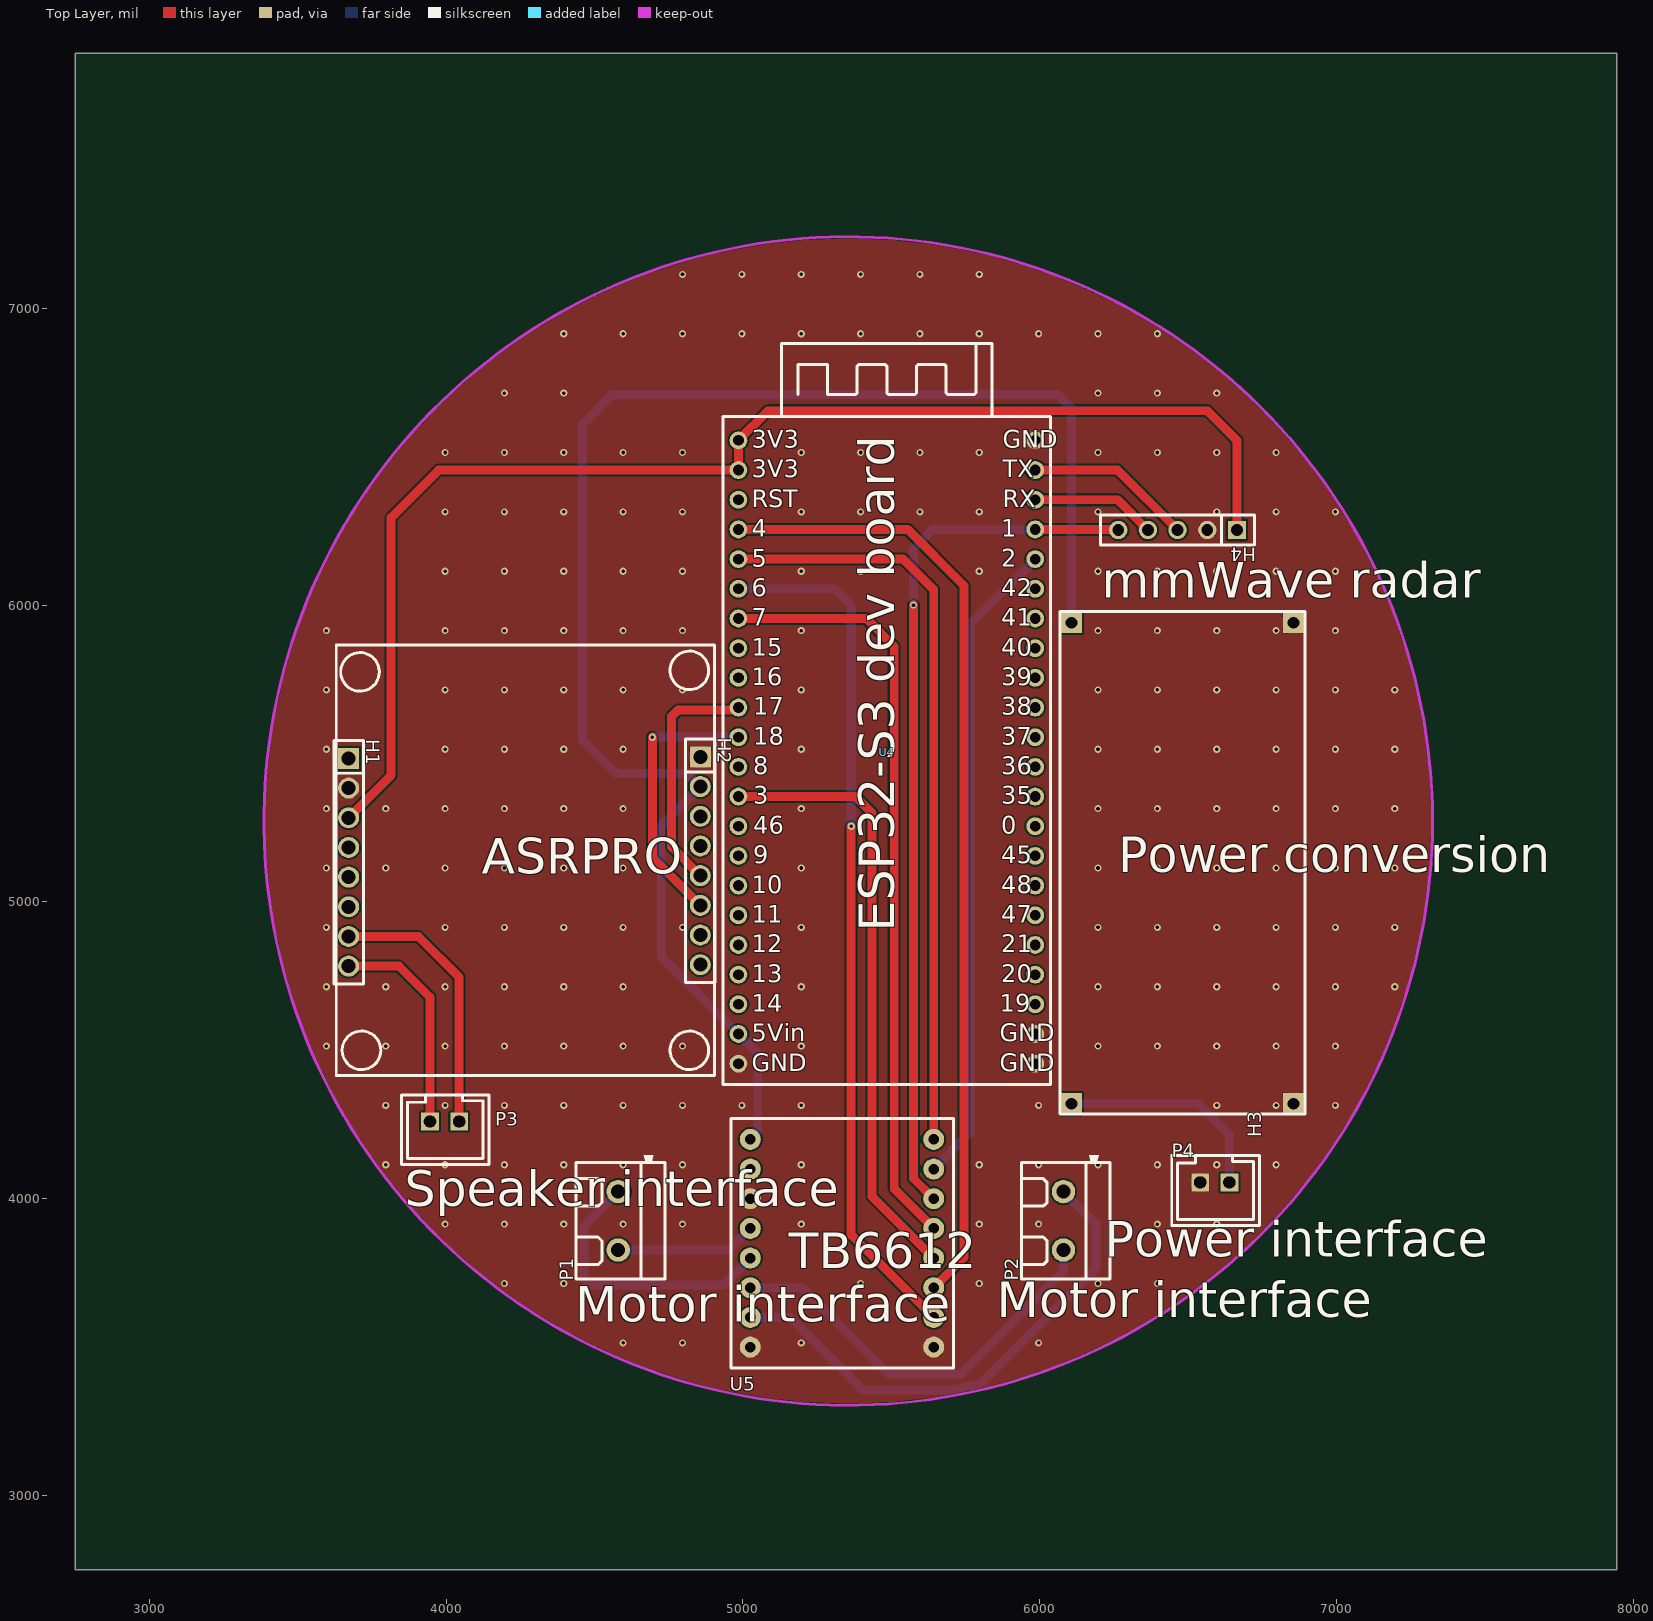
[diagram p0: Top Layer view]
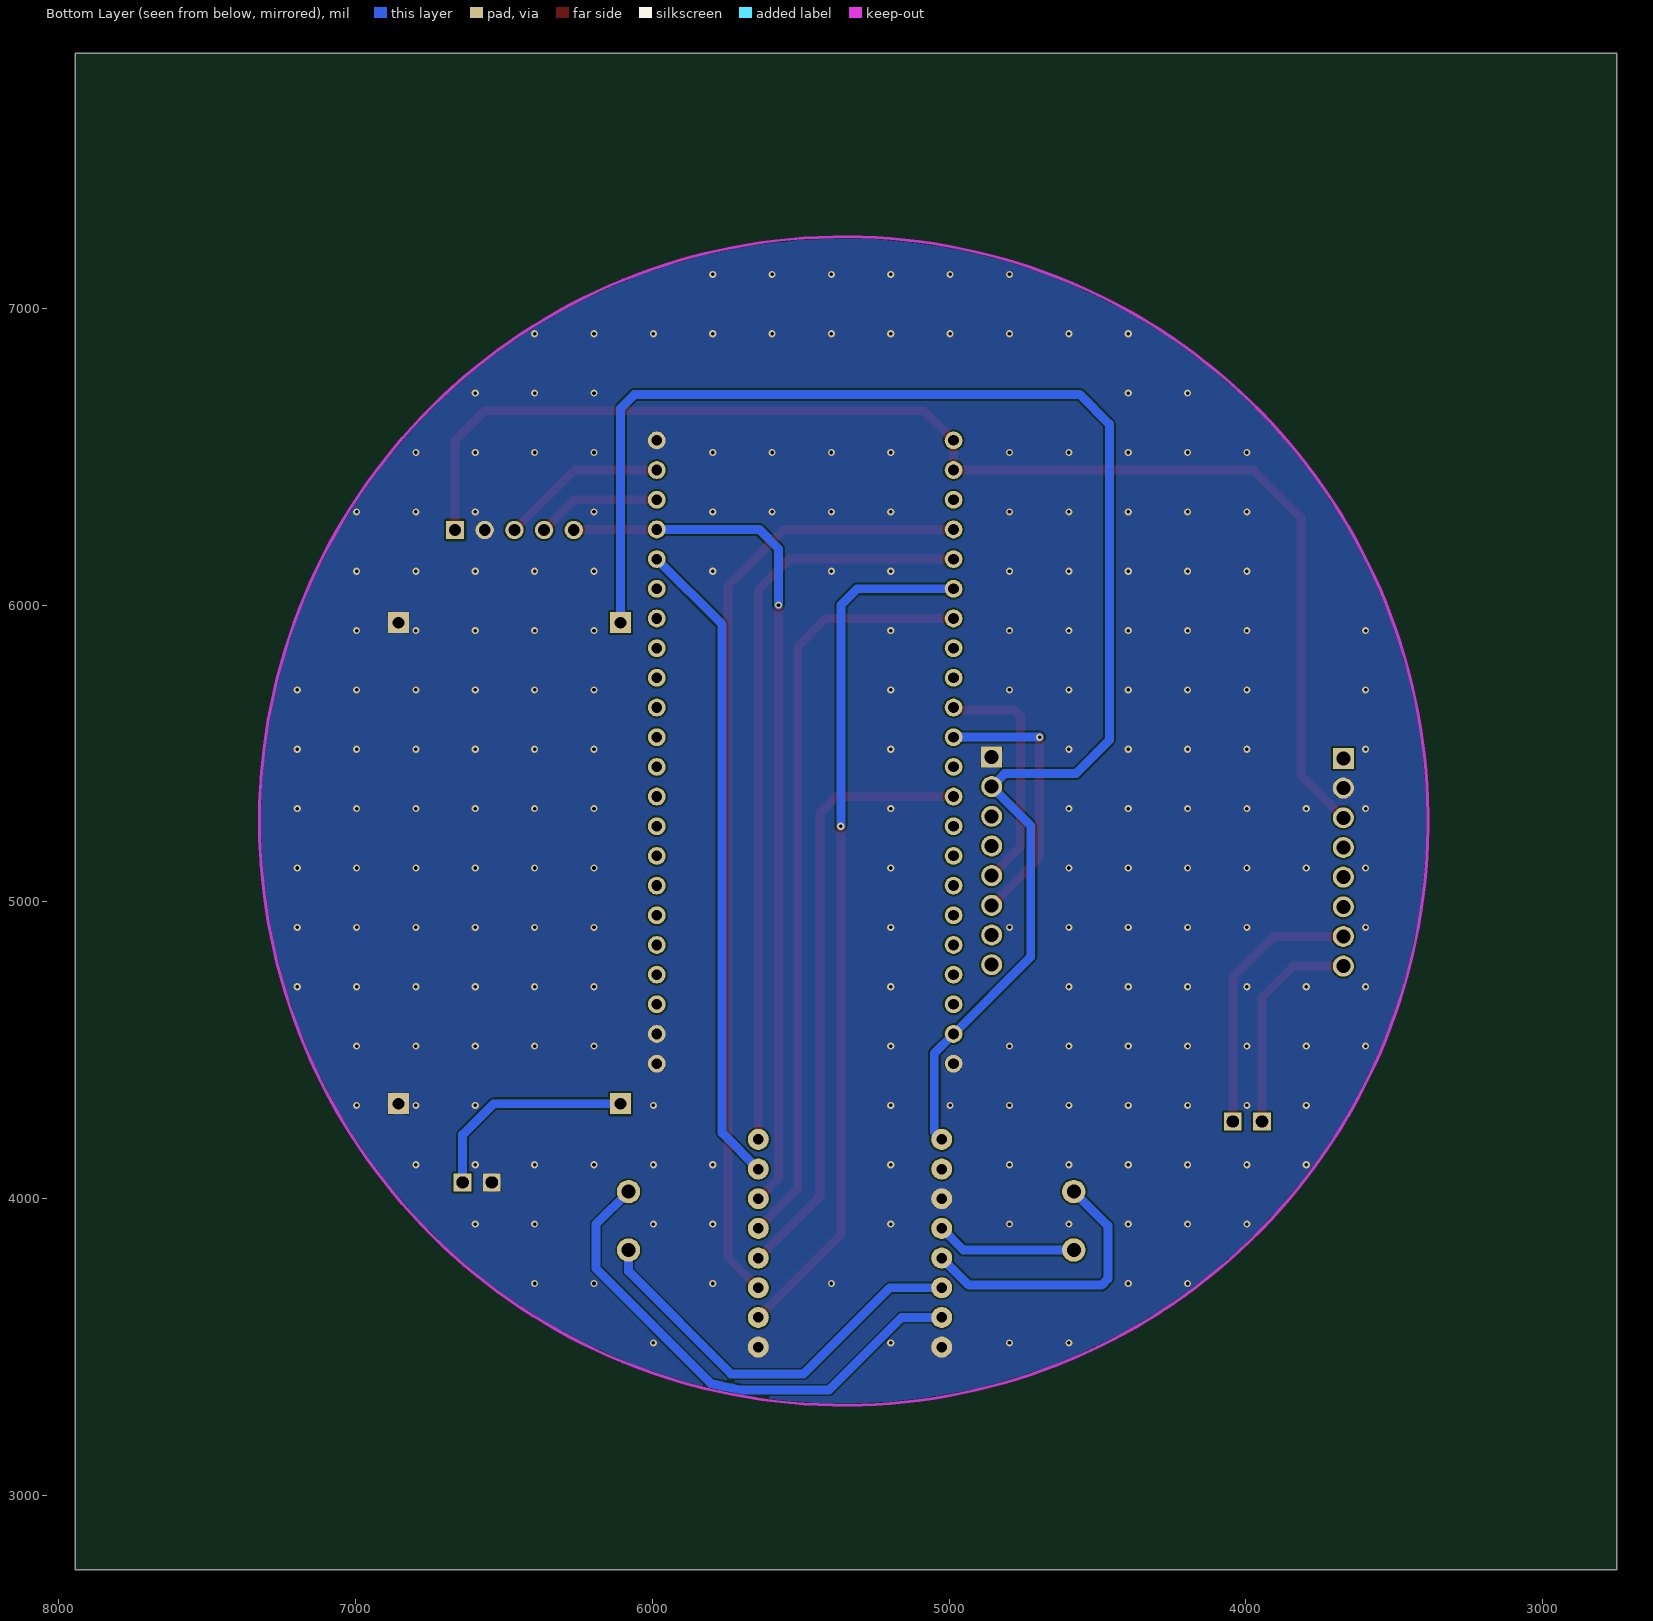
[diagram p1: Bottom Layer view, seen from below]
# Altium PCB MISC89096.pcbdoc
Units mil, origin at the board's own origin, x right, y up, seen from the top; angles counter-clockwise.
Board outline 5195 x 5110 mil, 2 copper layers (Top Layer, Bottom Layer), stack 62.206 mil thick; 10 components, 47 nets, 93 pads, 211 vias.

## Layer stack, top to bottom
Top Solder Mask Layer: solder mask 0.394, Dk 3.3
Top Layer: signal copper 1.379
Dielectric1: surface 59.449, FR4, Dk 4.5
Bottom Layer: signal copper 1.378
Bottom Solder Mask Layer: solder mask 0.394, Dk 3.3

## Board outline
7945,2750 2750,2750 2750,7860 7945,7860

## Design rules (kind name [scope] priority, off if disabled: settings)
BoardOutlineClearance Plane_Default_1 [All] p2 off: genericclearance=6 ignorepadtopadclearanceinfootprint=FALSE except(0: Arc-SplitContinuation Track-SplitContinuation SMDPad-SplitContinuation THPad-SplitContinuation Via-SplitContinuation Fill-SplitContinuation Region-SplitContinuation Poly-SplitContinuation Text-SplitContinuation Hole-SplitContinuation; 6: Arc-OutlineEdge Track-OutlineEdge SMDPad-OutlineEdge THPad-OutlineEdge Via-OutlineEdge Fill-OutlineEdge Region-OutlineEdge Poly-OutlineEdge Text-OutlineEdge Hole-OutlineEdge Arc-CutoutEdge Track-CutoutEdge SMDPad-CutoutEdge THPad-CutoutEdge Via-CutoutEdge Fill-CutoutEdge Region-CutoutEdge Poly-CutoutEdge Text-CutoutEdge Hole-CutoutEdge)
BoardOutlineClearance Copper_Default_1 [All] p4 off: genericclearance=6 ignorepadtopadclearanceinfootprint=FALSE except(0: Arc-SplitContinuation Track-SplitContinuation SMDPad-SplitContinuation THPad-SplitContinuation Via-SplitContinuation Fill-SplitContinuation Region-SplitContinuation Poly-SplitContinuation Text-SplitContinuation Hole-SplitContinuation; 6: Arc-OutlineEdge Track-OutlineEdge SMDPad-OutlineEdge THPad-OutlineEdge Via-OutlineEdge Fill-OutlineEdge Region-OutlineEdge Poly-OutlineEdge Text-OutlineEdge Hole-OutlineEdge Arc-CutoutEdge Track-CutoutEdge SMDPad-CutoutEdge THPad-CutoutEdge Via-CutoutEdge Fill-CutoutEdge Region-CutoutEdge Poly-CutoutEdge Text-CutoutEdge Hole-CutoutEdge)
BoardOutlineClearance Copper_gge24019_1 [All] p6 off: genericclearance=6 ignorepadtopadclearanceinfootprint=FALSE except(0: Arc-SplitContinuation Track-SplitContinuation SMDPad-SplitContinuation THPad-SplitContinuation Via-SplitContinuation Fill-SplitContinuation Region-SplitContinuation Poly-SplitContinuation Text-SplitContinuation Hole-SplitContinuation; 6: Arc-OutlineEdge Track-OutlineEdge SMDPad-OutlineEdge THPad-OutlineEdge Via-OutlineEdge Fill-OutlineEdge Region-OutlineEdge Text-OutlineEdge Hole-OutlineEdge Arc-CutoutEdge Track-CutoutEdge SMDPad-CutoutEdge THPad-CutoutEdge Via-CutoutEdge Fill-CutoutEdge Region-CutoutEdge Text-CutoutEdge Hole-CutoutEdge; 10: Poly-OutlineEdge Poly-CutoutEdge)
BoardOutlineClearance Default_1 [All] p8: genericclearance=6 ignorepadtopadclearanceinfootprint=FALSE except(0: Arc-SplitContinuation Track-SplitContinuation SMDPad-SplitContinuation THPad-SplitContinuation Via-SplitContinuation Fill-SplitContinuation Region-SplitContinuation Poly-SplitContinuation Text-SplitContinuation Hole-SplitContinuation; 6: Arc-OutlineEdge Track-OutlineEdge SMDPad-OutlineEdge THPad-OutlineEdge Via-OutlineEdge Fill-OutlineEdge Region-OutlineEdge Poly-OutlineEdge Text-OutlineEdge Hole-OutlineEdge Arc-CutoutEdge Track-CutoutEdge SMDPad-CutoutEdge THPad-CutoutEdge Via-CutoutEdge Fill-CutoutEdge Region-CutoutEdge Poly-CutoutEdge Text-CutoutEdge Hole-CutoutEdge)
Clearance Plane_Default [All] p1 off: gap=6 ignorepadtopadclearanceinfootprint=FALSE
Clearance Copper_Default [All] p3 off: gap=6 ignorepadtopadclearanceinfootprint=FALSE
Clearance Copper_gge24019 [All] p5 off: gap=6 ignorepadtopadclearanceinfootprint=FALSE except(10: Poly-Track Poly-SMDPad Poly-THPad Poly-Via Poly-Fill Poly-Region Poly-Poly Poly-Arc Poly-Text Poly-Hole)
Clearance Default [All] p7: gap=6 ignorepadtopadclearanceinfootprint=FALSE
DiffPairsRouting differentialPair [All] p1: maxlimit=6 minlimit=6 mostfreqgap=6 toplayer_minwidth=5 toplayer_prefwidth=10 toplayer_maxwidth=100 toplayer_mingap=6 toplayer_prefgap=6 toplayer_maxgap=6 bottomlayer_minwidth=5 bottomlayer_prefwidth=10 bottomlayer_maxwidth=100 bottomlayer_mingap=6 bottomlayer_prefgap=6 bottomlayer_maxgap=6 maxuncoupledlength=10
HoleToHoleClearance otherClearance [All] p1: gap=11.8 allowstackedmicrovias=TRUE
Length netLength [All] p1: minlimit=0 maxlimit=0
MatchedLengths netLengthTolerance [All] p1: tolerance=1000
PasteMaskExpansion Common [All] p1: expansion=0
PlaneConnect Default_4 [All] p1: planeconnectstyle=Relief reliefexpansion=20 reliefentries=4 reliefconductorwidth=0 reliefairgap=10
PolygonConnect gge24019 [All] p1 off: connectstyle=Relief reliefconductorwidth=0 reliefentries=4 polygonreliefangle="90 Angle" airgapwidth=1 smdpad.connectstyle=Relief smdpad.reliefconductorwidth=0 smdpad.reliefentries=4 smdpad.polygonreliefangle="90 Angle" smdpad.airgapwidth=10 via.connectstyle=Relief via.reliefconductorwidth=10 via.reliefentries=4 via.polygonreliefangle="90 Angle" via.airgapwidth=10
PolygonConnect Default_5 [All] p2: connectstyle=Relief reliefconductorwidth=0 reliefentries=4 polygonreliefangle="90 Angle" airgapwidth=1 smdpad.connectstyle=Relief smdpad.reliefconductorwidth=0 smdpad.reliefentries=4 smdpad.polygonreliefangle="90 Angle" smdpad.airgapwidth=10 via.connectstyle=Relief via.reliefconductorwidth=10 via.reliefentries=4 via.polygonreliefangle="90 Angle" via.airgapwidth=10
RoutingVias Default_3 [All] p1: holewidth=12 width=24 viastyle="Through Hole" minholewidth=12 minwidth=24 maxholewidth=2362 maxwidth=3938
SolderMaskExpansion Common_1 [IsVia] p1: expansion=-1000 istentingtop=TRUE
SolderMaskExpansion Common_1 [All] p2: expansion=2 istentingtop=FALSE
Width Default_2 [All] p1: maxlimit=10 minlimit=10 preferedwidth=10 toplayer_minwidth=10 toplayer_maxwidth=1000 toplayer_prefwidth=10 bottomlayer_minwidth=10 bottomlayer_maxwidth=1000 bottomlayer_prefwidth=10

## Components (designator, comment, footprint, x,y, rotation, side; value= is the part's Value field where it differs from the comment)
H1 "" HDR-TH_8P-P2.54-V-F-1 3671.85,5133.49 r270 top
H2 "" HDR-TH_8P-P2.54-V-F-1 4856.65,5138.49 r270 top
H3 "" HDR-TH_4P-P2.54-V-F-R2-C2-S2.54 6855,4320 r90 top
H4 "" HDR-TH_5P-P2.54-V-F 6464.74,6253.05 r180 top
P1 "KF301-2P terminal block" CONN-TH_XY301V-A-5.0-2P 4580,3925.64 r90 top
P2 "KF301-2P terminal block" CONN-TH_XY301V-A-5.0-2P 6080.18,3925.64 r90 top
P3 "XH2.54 straight socket-2P" CONN-TH_XH2.54-2P 3995,4260 r180 top
P4 "XH2.54 straight socket-2P" CONN-TH_XH2.54-2P 6590,4055 r180 top
U4 "NO" ESP32S3 5485,5510 r0 top
U5 "" tb6612 5025,4200 r0 top

## Footprints (in the part's own frame and the unit in brackets; to place one, negate y for a bottom-side part, rotate by r counter-clockwise, add the part's x,y. Pads: shape width x height; smd on the part's side, far side on the other; paste and mask are expansions set on the pad)
CONN-TH_XH2.54-2P [mil]
  rect 60x60 hole 39.37 slot 41.34 at 0 deg paste+0 mask+1.97: 1(-49.22,0) 2(49.21,0)
  silkscreen extent -150,-90 145,145
CONN-TH_XY301V-A-5.0-2P [mm]
  round 2 hole 1.2: 1(-2.5,0) 2(2.5,0)
  silkscreen extent -5,-4 5.6,3.6
ESP32S3 [mil]
  round 60 hole 36: 1(-500,-1055) 2(-500,-955) 3(-500,-855) 4(-500,-755) 5(-500,-655) 6(-500,-555) 7(-500,-455) 8(-500,-355) 9(-500,-255) 10(-500,-155) 11(-500,-55) 12(-500,45) 13(-500,145) 14(-500,245) 15(-500,345) 16(-500,445) 17(-500,545) 18(-500,645) 19(-500,745) 20(-500,845) 21(-500,945) 22(-500,1045) 23(500,-1055) 24(500,-955) 25(500,-855) 26(500,-755) 27(500,-655) 28(500,-555) 29(500,-455) 30(500,-355) 31(500,-255) 32(500,-155) 33(500,-55) 34(500,45) 35(500,145) 36(500,245) 37(500,345) 38(500,445) 39(500,545) 40(500,645) 41(500,745) 42(500,845) 43(500,945) 44(500,1045)
  silkscreen extent -551,-1126 551,1371
HDR-TH_4P-P2.54-V-F-R2-C2-S2.54 [mm]
  rect 1.8x1.8 hole 1: 1(0,19) 2(41.174,19) 3(0,0) 4(41.174,0)
  silkscreen extent -0.88,-1.01 42.12,19.99
HDR-TH_5P-P2.54-V-F [mil]
  rect 62x62 hole 40.16: 1(-200,0)
  round 62 hole 40.16: 2(-100,0) 3(0,0) 4(100,0) 5(200,0)
  silkscreen extent -260,-50 260,50
HDR-TH_8P-P2.54-V-F-1 [mm]
  rect 1.8x1.8 hole 1.2: 1(-8.89,0)
  round 1.8 hole 1.2: 2(-6.35,0) 3(-3.81,0) 4(-1.27,0) 5(1.27,0) 6(3.81,0) 7(6.35,0) 8(8.89,0)
  silkscreen extent -10.41,-1.25 10.41,1.25
tb6612 [mm]
  round 1.8 hole 0.9: 1(0,0) 2(0,-2.54) 3(0,-5.08) 4(0,-7.62) 5(0,-10.16) 6(0,-12.7) 7(0,-15.24) 8(0,-17.78) 9(15.697,-17.78) 10(15.697,-15.24) 11(15.697,-12.7) 12(15.697,-10.16) 13(15.697,-7.62) 14(15.697,-5.08) 15(15.697,-2.54) 16(15.697,0)
  silkscreen extent -1.65,-19.56 17.4,1.78

## Via types
v1: diameter 24, hole 12, Top Layer to Bottom Layer, 208 vias
v2: diameter 24.02, hole 12, Top Layer to Bottom Layer, 3 vias

## Nets (pads, with @x,y where several pads share a name; then routed paths per layer and width w, separated by ;. In a path a pad name is that pad's centre, name@x,y a point inside that pad or via, vN(x,y) a via of type N, cw(c..) or ccw(c..) an arc to the next point about the centre after c; other vN are vias at no path point)
0: U4.31
1: H4.5 U4.41 U5.14 | length 2935.6
  Top Layer w30: v2(5575,6000) 5575,4068 U5.14 ; U4.41 6262.79,6255 H4.5
  Bottom Layer w30: v2(5575,6000) 5575,6190 5640,6255 U4.41
2: U4.40 U5.15 | length 2196.7
  Bottom Layer w30: U5.15 5765,4222 5765,5935 U4.40
3: U4.10 U5.12 | length 2058.9
  Top Layer w30: U4.10 5380,5355 5435,5300 5435,4008 U5.12
4: U4.19 U5.11 | length 3246
  Top Layer w30: U4.19 5555,6255 5745,6065 5745,3802 U5.11
5: U4.18 U5.16 | length 2552.7
  Top Layer w30: U4.18 5540,6155 5643,6052 U5.16
6: U4.17 U5.10 | length 2917.9
  Top Layer w30: v2(5365,5255) 5365,3878 U5.10
  Bottom Layer w30: U4.17 5310,6055 5365,6000 v2(5365,5255)
7: U4.16 U5.13 | length 2579.4
  Top Layer w30: U4.16 5415,5955 5510,5860 5510,4033 U5.13
8: U4.11
9: U4.8
10: U4.7
11: U4.6
12: U4.5
12V: H3.1 P4.1 | length 736.2
  Bottom Layer w30: H3.1 6535,4320 6639.22,4215.78 P4.1
13: U4.4
14: U4.3
15: U4.15
16: U4.14
17: H2.5 U4.13 | length 814
  Top Layer w30: H2.5 4760,5185.14 4760,5625 4781.21,5646.21 4976.21,5646.21 U4.13
18: H2.6 U4.12 | length 923.5
  Top Layer w30: v2(4695,5555) 4695,5150.14 H2.6
  Bottom Layer w30: v2(4695,5555) U4.12
19: U4.25
20: U4.26
21: U4.27
35: U4.32
36: U4.33
37: U4.34
38: U4.35
39: U4.36
40: U4.37
41: U4.38
42: U4.39
45: U4.30
46: U4.9
47: U4.28
48: U4.29
$1N2406: P1.1 U5.4 | length 475.1
  Bottom Layer w30: P1.1 4952.21,3827.21 U5.4
$1N2407: P1.2 U5.5 | length 948.3
  Bottom Layer w30: P1.2 4465,3909.06 4465,3730 4486.21,3708.79 4933.79,3708.79 U5.5
$1N2408: P2.1 U5.6 | length 1390.3
  Bottom Layer w30: U5.6 5200,3700 5490,3410 5735,3410 6080.18,3755.18 P2.1
$1N2409: P2.2 U5.7 | length 1734
  Bottom Layer w30: U5.7 5160,3600 5405,3355 5694.87,3355 ccw(c5355,5272.61) 5802.14,3377.14 6190,3765 6190,3914.24 P2.2
$1N2428: H1.7 P3.1 | length 915.2
  Top Layer w30: H1.7 3906.51,4883.49 4044.22,4745.78 P3.1
$1N2429: H1.8 P3.2 | length 736.3
  Top Layer w30: H1.8 3841.51,4783.49 3945.78,4679.22 P3.2
+5V: H2.2 H3.2 U4.2 U5.1 | length 5344.3
  Bottom Layer w30: U5.1 5050,4225 5050,4490 U4.2 4725,4815 4725,5256.83 H2.2 4813.09,5432.05 4572.95,5432.05 4460,5545 4460,6610 4560,6710 6060,6710 6106.97,6663.03 H3.2
GND: H1.2 H2.1 H3.3 H3.4 H4.2 P4.2 U4.1 U4.23 U4.24 U4.44 U5.3 U5.8 U5.9
  other v1: 4596.6,3514.21 4796.6,3514.21 5196.6,3514.21 5996.6,3514.21 4196.6,3714.21 4396.6,3714.21 5396.6,3714.21 5796.6,3714.21 6196.6,3714.21 6396.6,3714.21 3996.6,3914.21 4196.6,3914.21 4396.6,3914.21 4596.6,3914.21 4796.6,3914.21 5196.6,3914.21 5796.6,3914.21 5996.6,3914.21 6396.6,3914.21 6596.6,3914.21 3796.6,4114.21 3996.6,4114.21 4196.6,4114.21 4396.6,4114.21 4596.6,4114.21 4796.6,4114.21 5196.6,4114.21 5796.6,4114.21 5996.6,4114.21 6196.6,4114.21 6396.6,4114.21 6596.6,4114.21 6796.6,4114.21 3796.6,4314.21 3996.6,4314.21 4196.6,4314.21 4396.6,4314.21 4596.6,4314.21 4796.6,4314.21 4996.6,4314.21 5196.6,4314.21 5996.6,4314.21 6596.6,4314.21 6796.6,4314.21 6996.6,4314.21 3596.6,4514.21 3796.6,4514.21 3996.6,4514.21 4196.6,4514.21 4396.6,4514.21 4596.6,4514.21 4796.6,4514.21 5196.6,4514.21 6196.6,4514.21 6396.6,4514.21 6596.6,4514.21 6796.6,4514.21 6996.6,4514.21 3596.6,4714.21 3796.6,4714.21 3996.6,4714.21 4196.6,4714.21 4396.6,4714.21 4596.6,4714.21 5196.6,4714.21 6196.6,4714.21 6396.6,4714.21 6596.6,4714.21 6796.6,4714.21 6996.6,4714.21 7196.6,4714.21 3596.6,4914.21 3996.6,4914.21 4196.6,4914.21 4396.6,4914.21 4596.6,4914.21 4796.6,4914.21 5196.6,4914.21 6196.6,4914.21 6396.6,4914.21 6596.6,4914.21 6796.6,4914.21 6996.6,4914.21 7196.6,4914.21 3596.6,5114.21 3796.6,5114.21 3996.6,5114.21 4196.6,5114.21 4396.6,5114.21 4596.6,5114.21 5196.6,5114.21 6196.6,5114.21 6396.6,5114.21 6596.6,5114.21 6796.6,5114.21 6996.6,5114.21 7196.6,5114.21 3596.6,5314.21 3796.6,5314.21 3996.6,5314.21 4196.6,5314.21 4396.6,5314.21 4596.6,5314.21 5196.6,5314.21 6196.6,5314.21 6396.6,5314.21 6596.6,5314.21 6796.6,5314.21 6996.6,5314.21 7196.6,5314.21 3596.6,5514.21 3996.6,5514.21 4196.6,5514.21 4396.6,5514.21 4596.6,5514.21 5196.6,5514.21 6196.6,5514.21 6396.6,5514.21 6596.6,5514.21 6796.6,5514.21 6996.6,5514.21 7196.6,5514.21 3596.6,5714.21 3996.6,5714.21 4196.6,5714.21 4396.6,5714.21 4596.6,5714.21 4796.6,5714.21 5196.6,5714.21 6196.6,5714.21 6396.6,5714.21 6596.6,5714.21 6796.6,5714.21 6996.6,5714.21 7196.6,5714.21 3596.6,5914.21 3996.6,5914.21 4196.6,5914.21 4396.6,5914.21 4596.6,5914.21 4796.6,5914.21 5196.6,5914.21 6196.6,5914.21 6396.6,5914.21 6596.6,5914.21 6796.6,5914.21 6996.6,5914.21 3996.6,6114.21 4196.6,6114.21 4396.6,6114.21 4596.6,6114.21 4796.6,6114.21 5196.6,6114.21 5396.6,6114.21 5796.6,6114.21 6196.6,6114.21 6396.6,6114.21 6596.6,6114.21 6796.6,6114.21 6996.6,6114.21 3996.6,6314.21 4196.6,6314.21 4396.6,6314.21 4596.6,6314.21 4796.6,6314.21 5196.6,6314.21 5396.6,6314.21 5596.6,6314.21 5796.6,6314.21 6196.6,6314.21 6596.6,6314.21 6796.6,6314.21 6996.6,6314.21 3996.6,6514.21 4196.6,6514.21 4396.6,6514.21 4596.6,6514.21 4796.6,6514.21 5196.6,6514.21 5396.6,6514.21 5596.6,6514.21 5796.6,6514.21 6196.6,6514.21 6396.6,6514.21 6596.6,6514.21 6796.6,6514.21 4196.6,6714.21 4396.6,6714.21 6196.6,6714.21 6396.6,6714.21 6596.6,6714.21 4396.6,6914.21 4596.6,6914.21 4796.6,6914.21 4996.6,6914.21 5196.6,6914.21 5396.6,6914.21 5596.6,6914.21 5796.6,6914.21 5996.6,6914.21 6196.6,6914.21 6396.6,6914.21 4796.6,7114.21 4996.6,7114.21 5196.6,7114.21 5396.6,7114.21 5596.6,7114.21 5796.6,7114.21
RST: U4.20
RX: H4.4 U4.42 | length 422
  Top Layer w30: U4.42 6262.79,6355 H4.4
TX: H4.3 U4.43 | length 563.4
  Top Layer w30: U4.43 6262.79,6455 H4.3
VCC: H1.3 H4.1 U4.21 U4.22 | length 4471.8
  Top Layer w30: H1.3 3815,5426.64 3815,6295 3975,6455 U4.21 U4.22 5085,6655 6565,6655 6664.74,6555.26 H4.1
pads on no net: H1.1 H1.4 H1.5 H1.6 H2.3 H2.4 H2.7 H2.8 U5.2

## Polygon pours and split planes (outlines as drawn)
GND on Top Layer (solid, remove dead copper, pour order 2): 3020,7565 3020,3000 7685,3000 7685,7565
GND on Bottom Layer (solid, remove dead copper, pour order 2): 3000,7610 3000,3140 7695,3140 7695,7610

## Keep-outs
Board Outline Layer:
  circle w10: c5355,5272.62 r1968.5

## Silkscreen, mask and mechanical layers (free items; w line width, h text height)
Top Silkscreen Layer:
  circle w10: c4820,5780 r65
  circle w10: c3710,5775 r65
  circle w10: c3715,4500 r65
  circle w10: c4820,4500 r65
  lines w10: 3630,4415 3630,5865 4905,5865 4905,4415 3630,4415
  text "mmWave radar" at 6210,6025 h120
  text "Power conversion" at 6265,5100 h120
  text "ASRPRO" at 4120,5095 h120
  text "ESP32-S3 dev board" at 5510,4900 h120 r90
  text "Speaker interface" at 3860,3975 h120
  text "Power interface" at 6220,3805 h120
  text "TB6612" at 5155,3765 h120
  text "Motor interface" at 5855,3600 h120
  text "Motor interface" at 4435,3585 h120